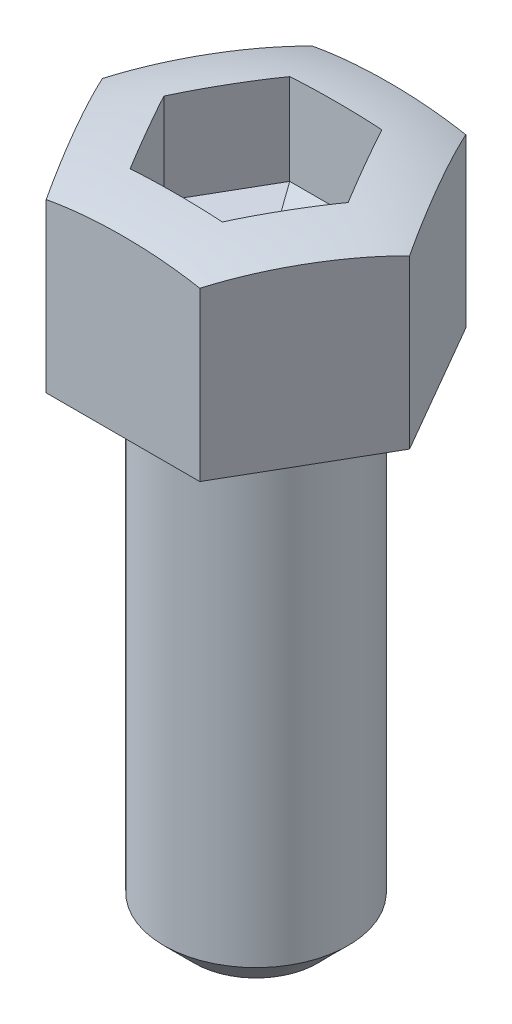
SolidWorks part; units mm, degrees
ref_plane "Front" through (0, 0, 0) normal (0, 0, 1) x (1, 0, 0)
ref_plane "Top" through (0, 0, 0) normal (0, 1, 0) x (1, 0, 0)
ref_plane "Right" through (0, 0, 0) normal (1, 0, 0) x (0, 0, -1)
sketch "Sketch1" plane through (0, 0, 0) normal (0, 0, 1) x (1, 0, 0)
  line L0 (0, 0) -> (3, 0)
  line L1 (3, 0) -> (3, 16)
  line L2 (3, 16) -> (5, 16)
  line L3 (5, 16) -> (5, 22)
  line L4 (5, 22) -> (0, 22)
  line L5 (0, 22) -> (0, 0.8125)
  line L6 (0, 0.8125) -> (0, 0)
  dimension "D1" = 3
  dimension "D2" = 16
  dimension "D3" = 2
  dimension "D4" = 6
revolve "Revolve1" add sketch "Sketch1" angle 360 about L5
sketch "Sketch2" plane through (0, 22, 0) normal (0, 1, 0) x (1, 0, 0)
  line L1 (5, 0) -> (2.5, 4.3301)
  line L2 (2.5, 4.3301) -> (-2.5, 4.3301)
  line L3 (-2.5, 4.3301) -> (-5, 0)
  line L4 (-5, 0) -> (-2.5, -4.3301)
  line L5 (-2.5, -4.3301) -> (2.5, -4.3301)
  line L6 (2.5, -4.3301) -> (5, 0)
  line L7 (-5.5082, 5.4719) -> (6.9262, 5.4719)
  line L8 (-5.5082, 5.4719) -> (-5.5082, -5.5809)
  line L9 (-5.5082, -5.5809) -> (6.9262, -5.5809)
  line L10 (6.9262, 5.4719) -> (6.9262, -5.5809)
  circle A0 centre (0, 0) radius 4.3301 construction
extrude "Cut-Extrude2" cut sketch "Sketch2" against normal up to surface (6 mm away) up to face at (0, 16, 5)
sketch "Sketch3" plane through (0, 22, 0) normal (0, 1, 0) x (1, 0, 0)
  line L1 (3, 0) -> (1.5, 2.5981)
  line L2 (1.5, 2.5981) -> (-1.5, 2.5981)
  line L3 (-1.5, 2.5981) -> (-3, 0)
  line L4 (-3, 0) -> (-1.5, -2.5981)
  line L5 (-1.5, -2.5981) -> (1.5, -2.5981)
  line L6 (1.5, -2.5981) -> (3, 0)
  circle A0 centre (0, 0) radius 2.5981 construction
  dimension "D1" = 6
extrude "Cut-Extrude3" cut sketch "Sketch3" against normal blind 3
sketch "Sketch4" plane through (0, 0, 0) normal (0, 0, 1) x (1, 0, 0)
  point P6 (0, 17.6856)
sketch "Sketch5" plane through (0, 19, 0) normal (0, 1, 0) x (1, 0, 0)
  line L0 (1.5, 2.5981) -> (-1.5, 2.5981) construction
  line L1 (1.5, 2.5981) -> (-1.5, 2.5981)
  line L2 (3, 0) -> (1.5, 2.5981) construction
  line L3 (3, 0) -> (1.5, 2.5981)
  line L4 (1.5, -2.5981) -> (3, 0) construction
  line L5 (1.5, -2.5981) -> (3, 0)
  line L6 (-1.5, -2.5981) -> (1.5, -2.5981) construction
  line L7 (-1.5, -2.5981) -> (1.5, -2.5981)
  line L8 (-3, 0) -> (-1.5, -2.5981) construction
  line L9 (-3, 0) -> (-1.5, -2.5981)
  line L10 (-1.5, 2.5981) -> (-3, 0) construction
  line L11 (-1.5, 2.5981) -> (-3, 0)
loft "Cut-Loft1" cut profiles "Sketch5", "Sketch4"
chamfer "Chamfer1" distance 1 angle 45 1 edges at (0, 0, 3)
sketch "Sketch6" plane through (0, 0, 0) normal (1, 0, 0) x (0, 0, -1)
  line L1 (-5.4645, 21.265) -> (-5.8879, 22.1697)
  line L2 (-5.8879, 22.1697) -> (-3.885, 23.6424)
  line L3 (-3.885, 23.6424) -> (-2.5981, 22)
  line L4 (0, 16) -> (0, 25.3448) construction
  line L5 (-3, 16) -> (3, 16) construction
  arc A0 (-2.5981, 22) -> (-5.4645, 21.265) centre (-1.7034, 12.5543) ccw
revolve "Cut-Revolve1" cut sketch "Sketch6" angle 360 about L4
